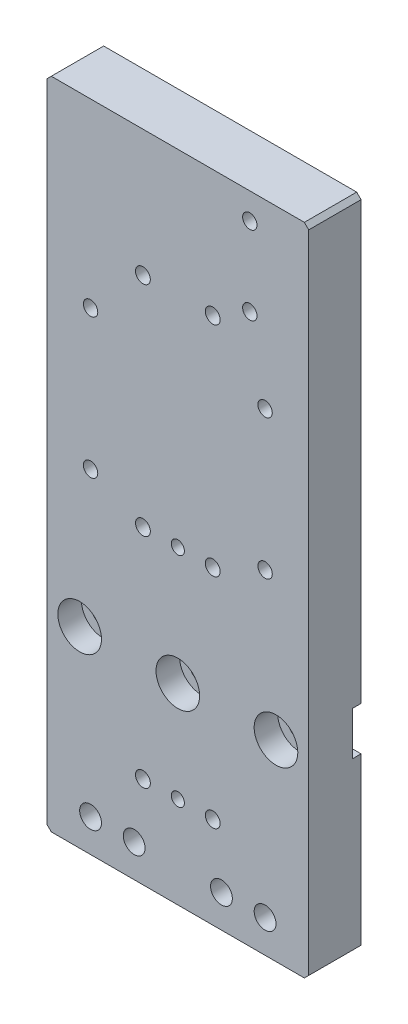
SolidWorks part; units mm, degrees
material "AL6061"
ref_plane "Front Plane" through (0, 0, 0) normal (0, 0, 1) x (1, 0, 0)
ref_plane "Top Plane" through (0, 0, 0) normal (0, 1, 0) x (1, 0, 0)
ref_plane "Right Plane" through (0, 0, 0) normal (1, 0, 0) x (0, 0, -1)
sketch "Sketch1" plane through (0, 0, 0) normal (0, 0, 1) x (1, 0, 0)
  line L1 (-30, 75) -> (30, 75)
  line L2 (-30, 75) -> (-30, -75)
  line L3 (-30, -75) -> (30, -75)
  line L4 (30, 75) -> (30, -75)
  line L5 (-30, 75) -> (30, -75) construction
  line L6 (-30, -75) -> (30, 75) construction
  point P0 (0, 0)
  dimension "D1" = 150
  dimension "D2" = 60
extrude "Boss-Extrude1" add sketch "Sketch1" along normal mid plane 12
hole_wizard "M4 Tapped Hole1" positions "Sketch4" profile "Sketch5" tap size "M4" standard "ISO" end condition through all
sketch "Sketch4" plane through (0, 0, -6) normal (0, 0, -1) x (-1, 0, 0)
  line L0 (-21, 71.3) -> (-13, 71.3) construction
  line L2 (-21, 53.3) -> (-13, 53.3) construction
  arc A0 (-13, 66.7) -> (-13, 71.3) centre (-13, 69) ccw construction
  point P0 (-16.5, 69)
  point P2 (-16.5, 51)
  dimension "D1" = 3.5
  dimension "D2" = 2.3
  dimension "D3" = 2.3
sketch "Sketch5" plane through (16.5, 69, -6) normal (1, 0, 0) x (0, 1, 0)
  line L0 (0, 0) -> (0, 12)
  line L1 (0, 12) -> (1.65, 12)
  line L2 (1.65, 12) -> (1.65, 0)
  line L5 (1.65, 0) -> (0, 0)
  line L11 (0, -6.35) -> (0, 107.95) construction
  dimension "通孔螺纹孔钻头直径" = 3.3
  dimension "通孔螺纹孔钻头深度" = 12
cosmetic thread "Cosmetic Thread1" parameters "D2"=4
cosmetic thread "Cosmetic Thread2" parameters "D2"=4
hole_wizard "CBORE for M4 Hex Socket Head Cap Screw1" positions "Sketch6" profile "Sketch7" counterbore size "M4" standard "ISO"
sketch "Sketch6" plane through (0, 0, -6) normal (0, 0, -1) x (-1, 0, 0)
  point P0 (-10, -9)
  point P3 (10, -9)
  point P6 (10, -29)
  point P9 (-10, -29)
  point P12 (10, -49)
  point P15 (-10, -49)
sketch "Sketch7" plane through (10, -9, -6) normal (1, 0, 0) x (0, 1, 0)
  line L0 (0, 0) -> (0, 12)
  line L1 (0, 12) -> (2.3, 12)
  line L3 (2.3, 12) -> (2.3, 4.4)
  line L4 (2.3, 4.4) -> (4, 4.4)
  line L5 (4, 4.4) -> (4, 0)
  line L7 (4, 0) -> (0, 0)
  line L11 (0, -6.35) -> (0, 107.95) construction
  dimension "通孔孔直径" = 4.6
  dimension "通孔孔深度" = 12
  dimension "柱形沉头孔直径" = 8
  dimension "柱形沉头孔深度" = 4.4
hole_wizard "M4 Tapped Hole2" positions "Sketch10" profile "Sketch11" tap size "M4" standard "ISO"
sketch "Sketch10" plane through (0, 0, -6) normal (0, 0, -1) x (-1, 0, 0)
  line L3 (24, 35.8) -> (16, 35.8) construction
  line L4 (24, -0.8) -> (16, -0.8) construction
  arc A2 (24, 31.2) -> (24, 35.8) centre (24, 33.5) ccw construction
  arc A3 (-16, 31.2) -> (-16, 35.8) centre (-16, 33.5) ccw construction
  point P0 (-20, 33.5)
  point P2 (-20, 1.5)
  point P4 (20, 33.5)
  point P6 (20, 1.5)
  dimension "D1" = 2.3
  dimension "D2" = 4
  dimension "D3" = 4
  dimension "D4" = 2.3
sketch "Sketch11" plane through (20, 33.5, -6) normal (1, 0, 0) x (0, 1, 0)
  line L0 (0, 0) -> (0, 16.4914)
  line L1 (0, 16.4914) -> (1.65, 15.5)
  line L2 (1.65, 15.5) -> (1.65, 0)
  line L5 (1.65, 0) -> (0, 0)
  line L10 (0, 16.4914) -> (-1.65, 15.5) construction
  line L11 (0, -6.35) -> (0, 107.95) construction
  dimension "螺纹孔钻头直径" = 3.3
  dimension "螺纹孔钻头深度" = 15.5
  dimension "导头角度" = 118
cosmetic thread "Cosmetic Thread3" parameters "D1"=12, "D2"=4
cosmetic thread "Cosmetic Thread4" parameters "D1"=12, "D2"=4
cosmetic thread "Cosmetic Thread5" parameters "D1"=12, "D2"=4
cosmetic thread "Cosmetic Thread6" parameters "D1"=12, "D2"=4
hole_wizard "M6 Tapped Hole1" positions "Sketch12" profile "Sketch13" tap size "M6" standard "ISO"
sketch "Sketch12" plane through (0, 0, -6) normal (0, 0, -1) x (-1, 0, 0)
  point P0 (20, -33)
  point P3 (-20, -33)
sketch "Sketch13" plane through (-20, -33, -6) normal (1, 0, 0) x (0, 1, 0)
  line L0 (0, 0) -> (0, 12)
  line L1 (0, 12) -> (2.5, 12)
  line L2 (2.5, 12) -> (2.5, 0)
  line L5 (2.5, 0) -> (0, 0)
  line L11 (0, -6.35) -> (0, 107.95) construction
  dimension "通孔螺纹孔钻头直径" = 5
  dimension "通孔螺纹孔钻头深度" = 12
cosmetic thread "Cosmetic Thread7" [suppressed] parameters "D2"=6
cosmetic thread "Cosmetic Thread8" [suppressed] parameters "D2"=6
hole_wizard "M6 Tapped Hole2" positions "Sketch14" profile "Sketch15" tap size "M6" standard "ISO" end condition through all
sketch "Sketch14" plane through (0, 0, -6) normal (0, 0, -1) x (-1, 0, 0)
  point P0 (20, -67.5)
  point P3 (-20, -67.5)
sketch "Sketch15" plane through (-20, -67.5, -6) normal (1, 0, 0) x (0, 1, 0)
  line L0 (0, 0) -> (0, 12)
  line L1 (0, 12) -> (2.5, 12)
  line L2 (2.5, 12) -> (2.5, 0)
  line L5 (2.5, 0) -> (0, 0)
  line L11 (0, -6.35) -> (0, 107.95) construction
  dimension "通孔螺纹孔钻头直径" = 5
  dimension "通孔螺纹孔钻头深度" = 12
cosmetic thread "Cosmetic Thread9" parameters "D2"=6
cosmetic thread "Cosmetic Thread10" parameters "D2"=6
hole_wizard "Blind Pin Hole2 size mm" positions "Sketch16" profile "Sketch17" hole size "Ø5.0" standard "ISO" end condition through all
sketch "Sketch16" plane through (0, 0, -6) normal (0, 0, -1) x (-1, 0, 0)
  point P0 (10, -67.5)
  point P3 (-10, -67.5)
sketch "Sketch17" plane through (-10, -67.5, -6) normal (1, 0, 0) x (0, 1, 0)
  line L0 (0, 0) -> (0, 12)
  line L1 (0, 12) -> (2.5, 12)
  line L2 (2.5, 12) -> (2.5, 0)
  line L5 (2.5, 0) -> (0, 0)
  line L11 (0, -6.35) -> (0, 107.95) construction
  dimension "通孔孔直径" = 5
  dimension "通孔孔深度" = 12
chamfer "Chamfer1" distance 1 angle 45 4 edges at (-30, -75, 0) (30, -75, 0) (30, 75, 0) (-30, 75, 0)
hole_wizard "CBORE for M3 Hex Socket Head Cap Screw1" positions "Sketch18" profile "Sketch19" counterbore size "M3" standard "ISO" end condition through all
sketch "Sketch18" plane through (0, 0, -6) normal (0, 0, -1) x (-1, 0, 0)
  line L0 (0, 75) -> (0, -75) construction
  line L1 (-29, 75) -> (29, 75) construction
  line L2 (29, -75) -> (-29, -75) construction
  point P12 (-8, -54)
  point P15 (8, -54)
  dimension "D1" = 16
  dimension "D2" = 21
sketch "Sketch19" plane through (-8, -54, -6) normal (1, 0, 0) x (0, 1, 0)
  line L0 (0, 0) -> (0, 12)
  line L1 (0, 12) -> (1.7, 12)
  line L3 (1.7, 12) -> (1.7, 3.4)
  line L4 (1.7, 3.4) -> (3.25, 3.4)
  line L5 (3.25, 3.4) -> (3.25, 0)
  line L7 (3.25, 0) -> (0, 0)
  line L11 (0, -6.35) -> (0, 107.95) construction
  dimension "通孔孔直径" = 3.4
  dimension "通孔孔深度" = 12
  dimension "柱形沉头孔直径" = 6.5
  dimension "柱形沉头孔深度" = 3.4
pattern_linear "LPattern1" count 3 spacing 50 along (0, 1, 0) of "CBORE for M3 Hex Socket Head Cap Screw1"
sketch "Sketch20" plane through (0, 0, -6) normal (0, 0, -1) x (-1, 0, 0)
  line L0 (-8, -4) -> (8, -4) construction
  line L1 (-8, -54) -> (8, -54) construction
  line L2 (0, -54) -> (0, -4) construction
  circle A0 centre (0, -4) radius 1.5
  circle A1 centre (0, -54) radius 1.5
  dimension "D1" = 3
extrude "Cut-Extrude1" cut sketch "Sketch20" against normal through all
sketch "Sketch21" plane through (0, 0, -6) normal (0, 0, -1) x (-1, 0, 0)
  line L0 (-30, -31) -> (30, -31) construction
  line L1 (-30, -74) -> (-30, 74) construction
  line L2 (0, -75) -> (0, 75) construction
  line L3 (29, -75) -> (-29, -75) construction
  line L4 (-29, 75) -> (29, 75) construction
  line L5 (30, 74) -> (30, -74) construction
  line L6 (-30, -26) -> (30, -26)
  line L7 (-30, -26) -> (-30, -36)
  line L8 (-30, -36) -> (30, -36)
  line L9 (30, -26) -> (30, -36)
  line L10 (-30, -26) -> (30, -36) construction
  line L11 (-30, -36) -> (30, -26) construction
  point P10 (0, -31)
  dimension "D1" = 44
  dimension "D2" = 10
extrude "Cut-Extrude2" cut sketch "Sketch21" against normal blind 2
hole_wizard "CBORE for M5 Hex Socket Head Cap Screw1" positions "Sketch22" profile "Sketch23" counterbore size "M5" standard "ISO" end condition through all
sketch "Sketch22" plane through (0, 0, 6) normal (0, 0, 1) x (1, 0, 0)
  line L0 (-30, -31) -> (30, -31) construction
  line L1 (-30, 74) -> (-30, -74) construction
  line L2 (30, -74) -> (30, 74) construction
  line L5 (-29, -75) -> (29, -75) construction
  line L6 (0, -75) -> (0, 7.4634) construction
  point P20 (0, -31)
  point P22 (-22.5, -31)
  point P25 (22.5, -31)
  dimension "D1" = 44
  dimension "D2" = 45
sketch "Sketch23" plane through (22.5, -31, 6) normal (1, 0, 0) x (0, -1, 0)
  line L0 (0, 0) -> (0, 12)
  line L1 (0, 12) -> (2.75, 12)
  line L3 (2.75, 12) -> (2.75, 5.4)
  line L4 (2.75, 5.4) -> (5, 5.4)
  line L5 (5, 5.4) -> (5, 0)
  line L7 (5, 0) -> (0, 0)
  line L11 (0, -6.35) -> (0, 107.95) construction
  dimension "通孔孔直径" = 5.5
  dimension "通孔孔深度" = 12
  dimension "柱形沉头孔直径" = 10
  dimension "柱形沉头孔深度" = 5.4
